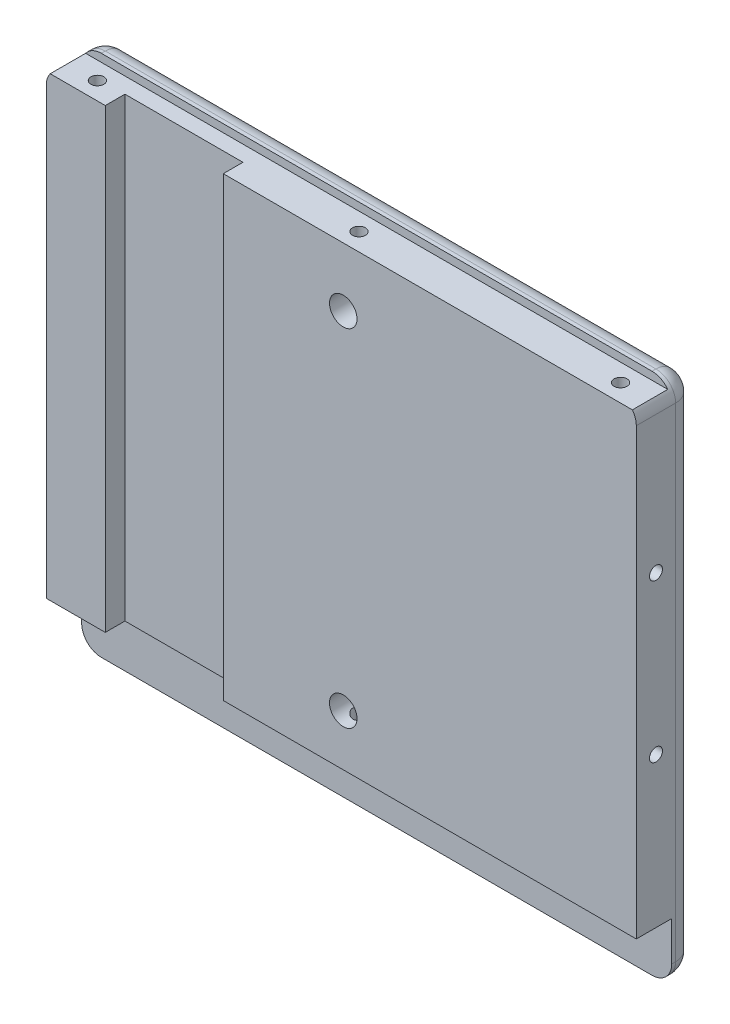
from build123d import *

# Parameters (mm, degrees)
SKETCH_1_W                  = 150
SKETCH_1_H                  = 133
EXTRUDE_1_DEPTH             = 15
SKETCH_2_W                  = 23.680798508
SKETCH_2_H                  = 30.226028772
CUT_EXTRUDE_1_DEPTH         = 165.764225486
FILLET_2_R                  = 5
HOLE_WIZARD_2_D             = 7
HOLE_WIZARD_2_CBORE_D       = 11
HOLE_WIZARD_2_CBORE_DEPTH   = 7
SKETCH_19_W                 = 244.102436516
SKETCH_19_H                 = 114.665953459
CUT_EXTRUDE_7_DEPTH         = 15
SKETCH_29_W                 = 30
SKETCH_29_H                 = 229.451153657
CUT_EXTRUDE_11_DEPTH        = 5
HOLE_WIZARD_M4_1_D          = 3.3
HOLE_WIZARD_M4_1_DEPTH      = 12
HOLE_WIZARD_M4_1_TIP        = 0.991420021
HOLE_WIZARD_M4_2_D          = 3.3
HOLE_WIZARD_M4_2_DEPTH      = 12
HOLE_WIZARD_M4_2_TIP        = 0.991420021
HOLE_WIZARD_M4_3_AT_2_COUNT = 2
HOLE_WIZARD_M4_3_AT_2_PITCH = 40


with BuildPart() as part:
    # 草图1 → 凸台-拉伸1 (new body)
    with BuildSketch(Plane.XY):
        Rectangle(SKETCH_1_W, SKETCH_1_H)
    extrude(amount=EXTRUDE_1_DEPTH)

    # 草图2 → 切除-拉伸1 (cut, through all)
    with BuildSketch(Plane.ZY.offset(75)):
        with Locations((17.840399254, 79.613014386)):
            Rectangle(SKETCH_2_W, SKETCH_2_H)
    extrude(amount=-CUT_EXTRUDE_1_DEPTH, mode=Mode.SUBTRACT)

    # 圆角2
    fillet_2_edges = [part.edges().sort_by_distance(p)[0] for p in [
        (-75, 66.5, 3),
        (-75, 0, 0),
        (-75, -66.5, 7.5),
        (0, -66.5, 0),
        (75, -66.5, 7.5),
        (75, 0, 0),
        (75, 66.5, 3),
        (0, 66.5, 0),
    ]]
    fillet(fillet_2_edges, radius=FILLET_2_R)

    # 打孔尺寸(%根据)开槽圆柱头螺钉的类型2 (through all)
    with Locations(Plane(origin=(0, 0, 0), x_dir=(-1, 0, 0), z_dir=(0, 0, -1))):
        with Locations((-0.5, 49.5), (-0.5, -38.5)):
            CounterBoreHole(HOLE_WIZARD_2_D / 2, HOLE_WIZARD_2_CBORE_D / 2, HOLE_WIZARD_2_CBORE_DEPTH)

    # 草图19 → 切除-拉伸7 (cut)
    with BuildSketch(Plane.XZ.offset(66.5)):
        with Locations((-15.450751356, 63.33297673)):
            Rectangle(SKETCH_19_W, SKETCH_19_H)
    extrude(amount=-CUT_EXTRUDE_7_DEPTH, mode=Mode.SUBTRACT)

    # 草图29 → 切除-拉伸11 (cut)
    with BuildSketch(Plane.XY.offset(15)):
        with Locations((-45, 14.041040746)):
            Rectangle(SKETCH_29_W, SKETCH_29_H)
    extrude(amount=-CUT_EXTRUDE_11_DEPTH, mode=Mode.SUBTRACT)

    # M4 螺纹孔1
    with Locations(Plane(origin=(0, -51.5, 0), x_dir=(-1, 0, 0), z_dir=(0, -1, 0))):
        with Locations((66.5, -10.5), (-66.5, -10.5), (0, -10.5)):
            Hole(HOLE_WIZARD_M4_1_D / 2, depth=HOLE_WIZARD_M4_1_DEPTH)
            with Locations((0, 0, -(HOLE_WIZARD_M4_1_DEPTH + HOLE_WIZARD_M4_1_TIP / 2))):  # 118° drill point
                Cone(0, HOLE_WIZARD_M4_1_D / 2, HOLE_WIZARD_M4_1_TIP, mode=Mode.SUBTRACT)

    # M4 螺纹孔2
    with Locations(Plane(origin=(0, 64.5, 0), x_dir=(1, 0, 0), z_dir=(0, 1, 0))):
        with Locations((-66.5, -10.5), (66.5, -10.5), (0, -10.5)):
            Hole(HOLE_WIZARD_M4_2_D / 2, depth=HOLE_WIZARD_M4_2_DEPTH)
            with Locations((0, 0, -(HOLE_WIZARD_M4_2_DEPTH + HOLE_WIZARD_M4_2_TIP / 2))):  # 118° drill point
                Cone(0, HOLE_WIZARD_M4_2_D / 2, HOLE_WIZARD_M4_2_TIP, mode=Mode.SUBTRACT)

    # 草图37 → M4 螺纹孔3 (revolve, cut)
    with BuildSketch(Plane(origin=(-75, 26.61076125, 10), x_dir=(0, 0, 1), z_dir=(0, 1, 0))):
        Polygon((0, 0), (0, 12.991420021), (1.65, 12), (1.65, 0), align=None)
    hole_wizard_m4_3 = revolve(axis=Axis((-81.35, 26.61076125, 10), (1, 0, 0)), mode=Mode.SUBTRACT)

    # M4 螺纹孔3 at 2: M4 螺纹孔3 ×2
    with Locations(*[(0, -i * HOLE_WIZARD_M4_3_AT_2_PITCH, 0) for i in range(1, HOLE_WIZARD_M4_3_AT_2_COUNT)]):
        add(hole_wizard_m4_3, mode=Mode.SUBTRACT)

    # 镜向1: M4 螺纹孔3 across plane
    add(hole_wizard_m4_3.mirror(Plane(origin=(0, 0, 0), x_dir=(0, 0, 1), z_dir=(1, 0, 0))), mode=Mode.SUBTRACT)

    # 镜向1 copy 1 sketch → 镜向1 copy 1 (revolve, cut)
    with BuildSketch(Plane(origin=(75, -13.38923875, 10), x_dir=(0, 0, 1), z_dir=(0, 1, 0))):
        Polygon((0, 0), (0, -12.991420021), (1.65, -12), (1.65, 0), align=None)
    revolve(axis=Axis((81.35, -13.38923875, 10), (1, 0, 0)), mode=Mode.SUBTRACT)


solid = part.part
